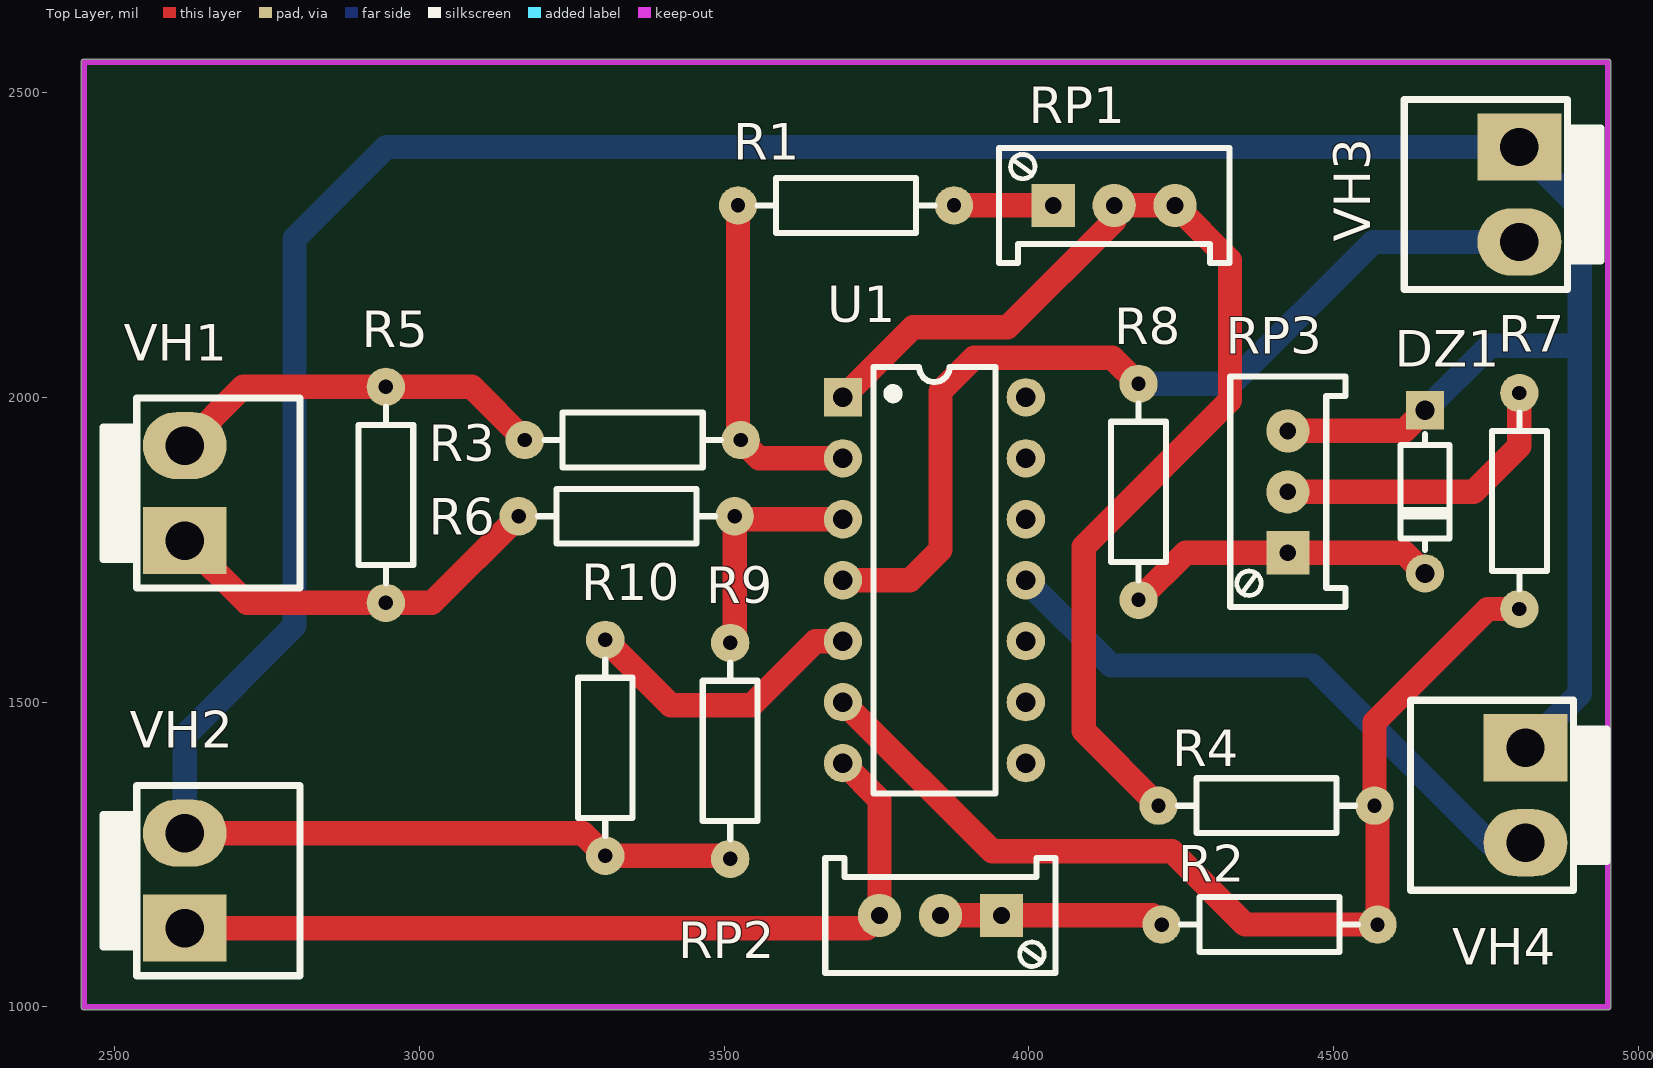
[diagram p0: Top Layer view]
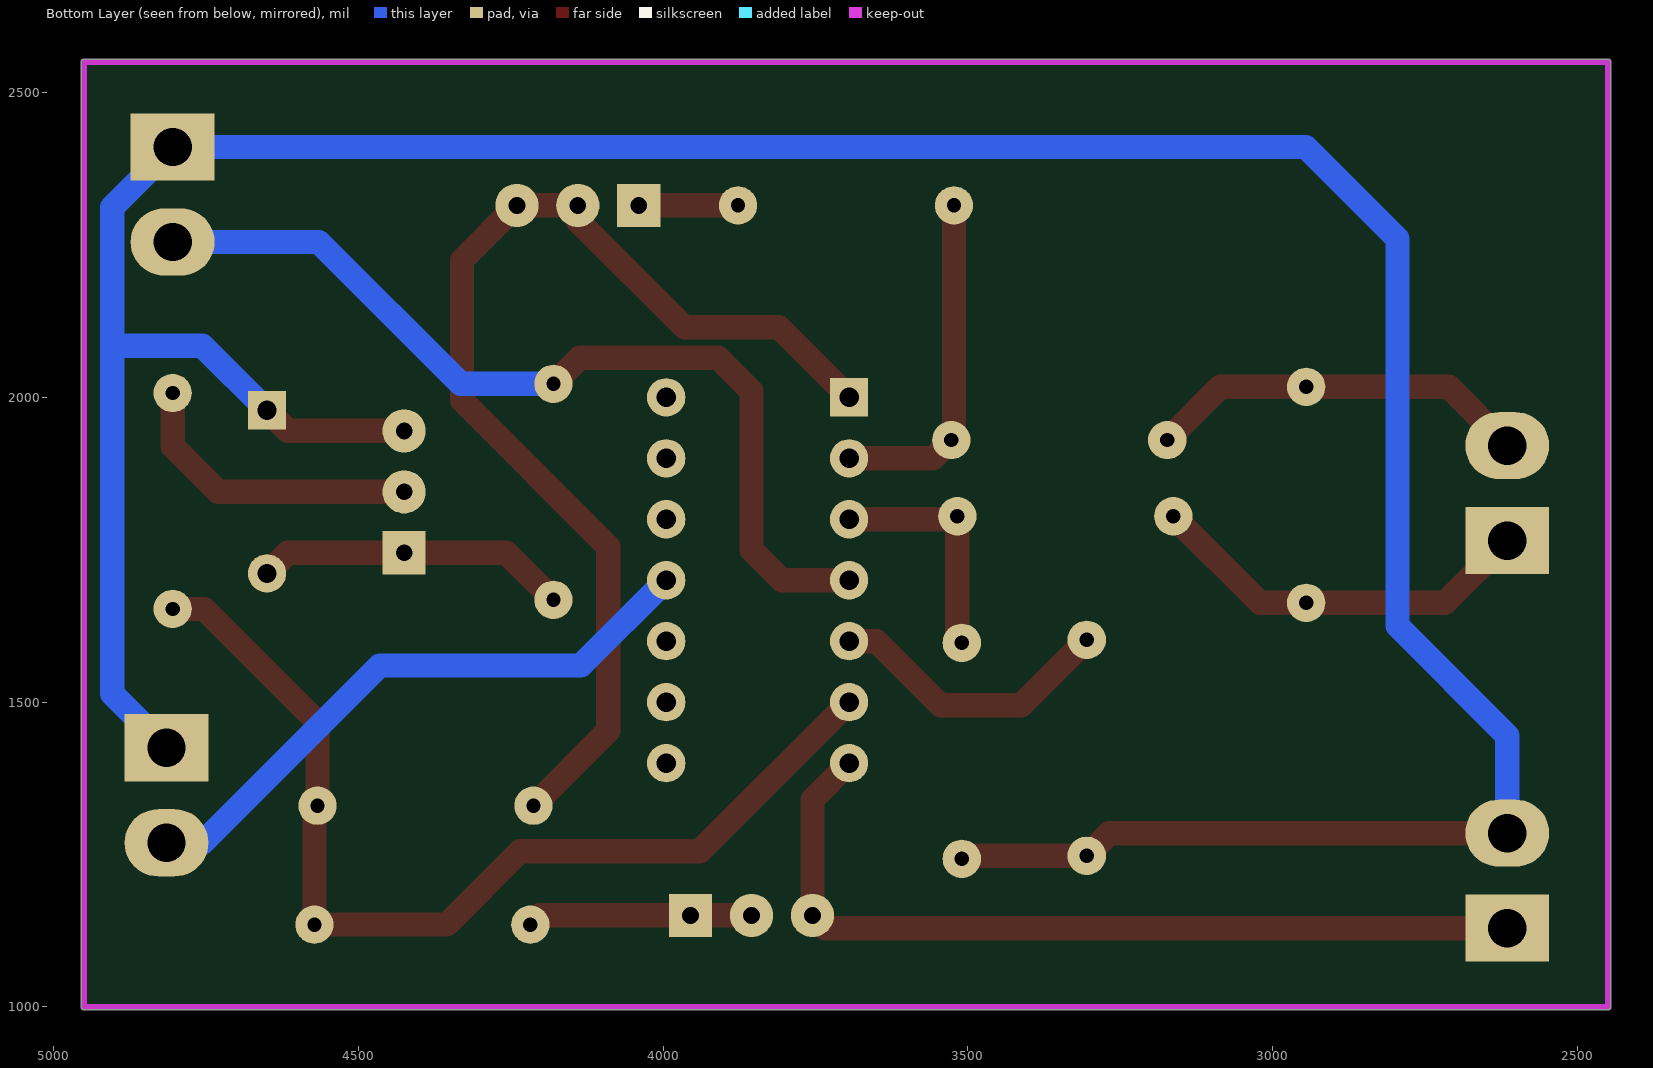
[diagram p1: Bottom Layer view, seen from below]
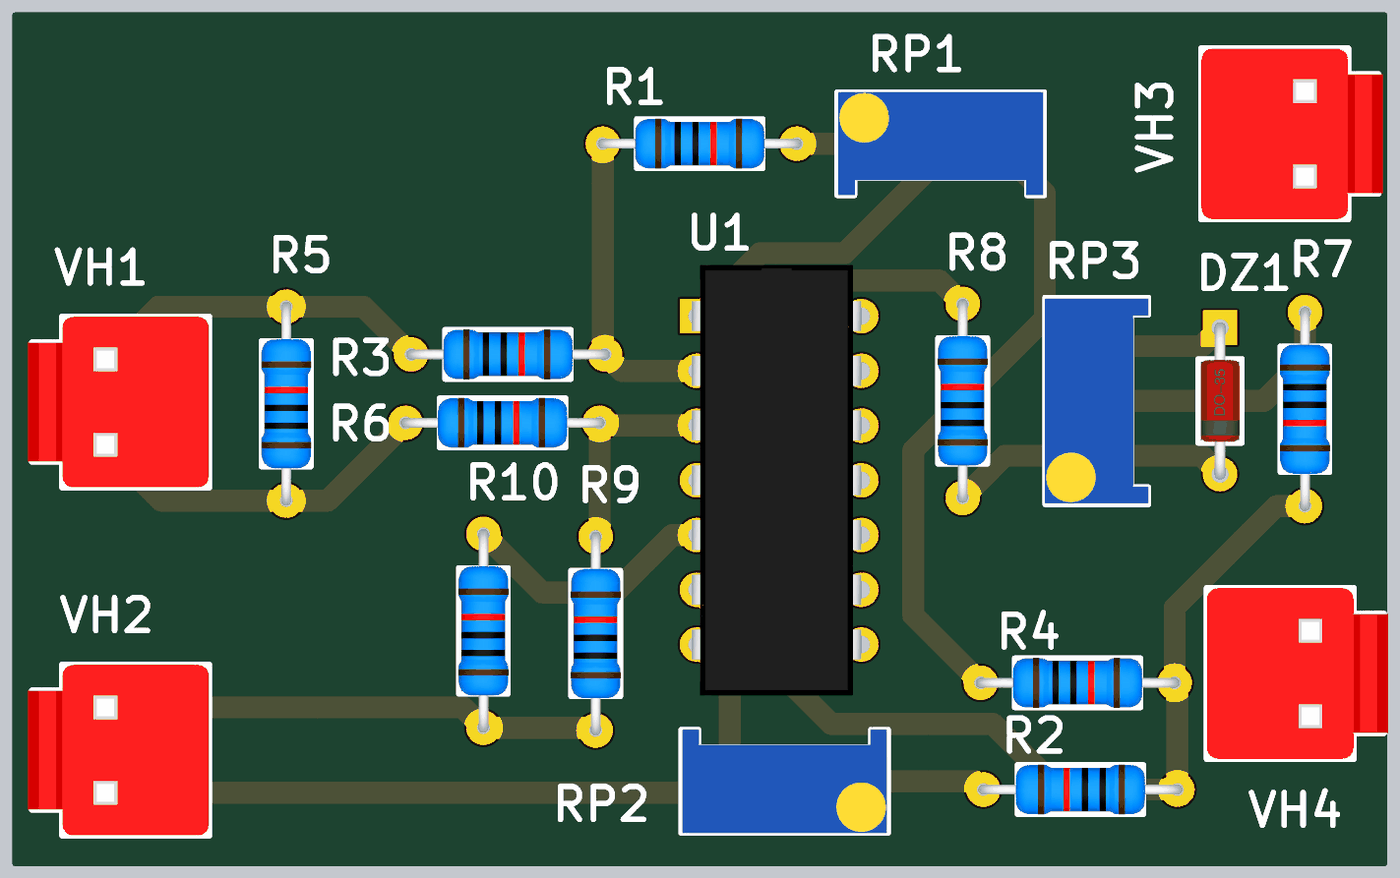
[diagram p2: 3D render of the assembled board from above, using the file's embedded part models]
# Altium PCB MISC80720.PcbDoc
Units mil, origin at the board's own origin, x right, y up, seen from the top; angles counter-clockwise.
Board outline 2510.03 x 1560.03 mil, 2 copper layers (Top Layer, Bottom Layer); 19 components, 15 nets, 53 pads, 0 vias.

## Layer stack, top to bottom (the 12.6 mil dielectric is the usual default, probably not edited)
Top Solder: solder mask 0.4, Solder Resist, Dk 3.5
Top Layer: signal copper 1.4
Dielectric 1: dielectric 12.6, FR-4, Dk 4.8
Bottom Layer: signal copper 1.4
Bottom Solder: solder mask 0.4, Solder Resist, Dk 3.5

## Board outline
2444.99,1000 ccw(c2450,1000) 2450,994.99 4950,994.99 ccw(c4950,1000) 4955.02,1000 4955.02,2550 ccw(c4950,2550) 4950,2555.01 2450,2555.01 ccw(c2450,2550) 2444.99,2550

## Design rules (kind name [scope] priority, off if disabled: settings)
Clearance [All] p1: gap=10
MinimumSolderMaskSliver [All] p1: minsoldermaskwidth=0
PolygonConnect [All] p1: connectstyle=Relief reliefconductorwidth=10 reliefentries=4 polygonreliefangle="90 Angle" airgapwidth=10
RoutingVias [All] p1: holewidth=28 width=50 viastyle="Through Hole" minholewidth=28 minwidth=50 maxholewidth=28 maxwidth=50
SilkToSilkClearance [All] p1: silktosilkclearance=0
SilkToSolderMaskClearance [IsPad] p1: minsilkscreentomaskgap=0 clearancetoexposedcopper=TRUE
SolderMaskExpansion [All] p1: expansion=4
Width [All] p1: maxlimit=40 minlimit=40 preferedwidth=40
27 further rules are at their usual default settings.

## Components (designator, comment, footprint, x,y, rotation, side; value= is the part's Value field where it differs from the comment)
DZ1 "6V2" DO-35 4650,1845 r270 top
R1 "9.1K" "RS 1/4W" 3700,2315 r0 top
R2 "22K" "RS 1/4W" 4395,1135 r180 top
R3 "10K" "RS 1/4W" 3350,1930 r0 top
R4 "10K" "RS 1/4W" 4390,1330 r0 top
R5 "500" "RS 1/4W" 2945,1840 r90 top
R6 "10K" "RS 1/4W" 3340,1805 r0 top
R7 "10K" "RS 1/4W" 4805,1830 r270 top
R8 "750" "RS 1/4W" 4180,1845 r90 top
R9 "10K" "RS 1/4W" 3510,1420 r90 top
R10 "3.9K" "RS 1/4W" 3305,1425 r90 top
RP1 "2K" 3296W 4140,2315 r0 top
RP2 "5K" 3296W 3855,1150 r180 top
RP3 "2K" 3296W 4425,1845 r90 top
U1 "LM124AD" DIP14 3695,2000 r0 top
VH1 "VH2" VH3.96-2A 2615,1765 r90 top
VH2 "VH2" VH3.96-2A 2615,1129.09 r90 top
VH3 "VH2" VH3.96-2A 4805,2410.91 r270 top
VH4 "VH2" VH3.96-2A 4815,1425 r270 top

## Footprints (in the part's own frame and the unit in brackets; to place one, negate y for a bottom-side part, rotate by r counter-clockwise, add the part's x,y. Pads: shape width x height; smd on the part's side, far side on the other; paste and mask are expansions set on the pad)
3296W [mm] "Precise Multi-Winding Adjustable Resistor"
  rect 1.8x1.8 hole 0.7: 1(-2.54,0)
  round 1.8 hole 0.7: 2(0,0) 3(2.54,0)
  silkscreen extent -4.8,-2.4 4.8,2.4, body extent -4.75,-2.4 4.75,2.4, height 11.52
DIP14 [mm]
  rect 1.6x1.6 hole 0.813: 1(0,0)
  round 1.6 hole 0.813: 2(0,-2.54) 3(0,-5.08) 4(0,-7.62) 5(0,-10.16) 6(0,-12.7) 7(0,-15.24) 8(7.62,-15.24) 9(7.62,-12.7) 10(7.62,-10.16) 11(7.62,-7.62) 12(7.62,-5.08) 13(7.62,-2.54) 14(7.62,0)
  silkscreen extent 1.27,-16.51 6.35,1.27, body extent -0.25,-17.62 7.62,2.38, height 5.1
DO-35 [mm] "1.8*6.8mm(直径，脚距）"
  rect 1.6x1.6 hole 0.8: 1(-3.4,0)
  round 1.6 hole 0.8: 2(3.4,0)
  silkscreen extent -2.41,-1.02 2.41,1.02, body extent -3.65,-0.9 3.65,0.9, height 1.85
"RS 1/4W" [mm] "直插色环电阻，脚距9mm，直径2.3mm"
  round 1.6 hole 0.6: 1(-4.5,0) 2(4.5,0)
  silkscreen extent -3.68,-1.14 3.68,1.14, body extent -4.72,-1.16 4.73,1.16, height 2.32
VH3.96-2A [mm]
  rect 2.8x3.5 hole 1.6: 1(0,0)
  oval 2.8x3.5 hole 1.6: 2(3.96,0)
  silkscreen extent -1.98,-4.8 5.94,3.4, body extent -1.98,-4.8 5.94,3.6, height 14.6

## Part data
DZ1: library part 1N4106, "12V/0.5W Zener diode"
R1 R2 R3 R4 R5 R6 R7 R8 R9 R10: library part R-S, "Color-band resistor"
RP1 RP2 RP3: library part RP, "Single-gang potentiometer"
U1: "Low-Power Quad Operational Amplifier"

## Nets (pads, with @x,y where several pads share a name; then routed paths per layer and width w, separated by ;. In a path a pad name is that pad's centre, name@x,y a point inside that pad or via, vN(x,y) a via of type N, cw(c..) or ccw(c..) an arc to the next point about the centre after c; other vN are vias at no path point)
+12V: R8.2 U1.4 VH3.2 | length 1527.7
  Top Layer w40: U1.4 3805,1700 3855,1750 3855,2010 3910,2065 4137.17,2065 R8.2
  Bottom Layer w40: R8.2 4332.17,2022.17 4565,2255 VH3.2
-12V: U1.11 VH4.2 | length 998.5
  Bottom Layer w40: U1.11 4135,1560 4465,1560 4755.91,1269.09 VH4.2
GND: DZ1.1 R9.1 R10.1 RP3.3 VH2.2 VH3.1 VH4.1 | length 5635.1
  Top Layer w40: VH2.2 3267.83,1285 R10.1 3505,1247.83 R9.1 ; RP3.3 4616.14,1945 DZ1.1
  Bottom Layer w40: VH2.2 2615,1445 2795,1625 2795,2260 2945.91,2410.91 VH3.1 4903.9,2312.01 4903.9,2085 ; DZ1.1 4756.14,2085 4903.9,2085 ; VH4.1 4903.9,1513.9 4903.9,2085
NetDZ1_2: DZ1.2 R8.1 RP3.1 | length 516
  Top Layer w40: R8.1 4257.17,1745 RP3.1 4616.14,1745 DZ1.2
NetR1_1: R1.1 R3.2 U1.2 | length 567.1
  Top Layer w40: R1.1 3522.83,1934.33 R3.2 3557.17,1900 U1.2
NetR1_2: R1.2 RP1.1 | length 162.8
  Top Layer w40: R1.2 RP1.1
NetR2_1: R2.1 R4.2 R7.2 U1.6 | length 1677.3
  Top Layer w40: U1.6 3940,1255 4235,1255 4355,1135 R2.1 4572.17,1325 R4.2 4567.17,1467.17 4752.83,1652.83 R7.2
NetR2_2: R2.2 RP2.1 RP2.2 | length 369
  Top Layer w40: RP2.2 RP2.1 4202.83,1150 R2.2
NetR3_1: R3.1 R5.2 VH1.2 | length 633.8
  Top Layer w40: VH1.2 2711.26,2017.17 R5.2 3085.67,2017.17 R3.1
NetR4_1: R4.1 RP1.2 RP1.3 U1.1 | length 1862.7
  Top Layer w40: U1.1 3810,2115 3965,2115 4140,2290 RP1.2 RP1.3 4330,2225 4330,1995 4090,1755 4090,1452.83 R4.1
NetR5_1: R5.1 R6.1 VH1.1 | length 649
  Top Layer w40: VH1.1 2717.17,1662.83 R5.1 3020.67,1662.83 R6.1
NetR6_2: R6.2 R9.2 U1.3 | length 390.7
  Top Layer w40: R9.2 3517.17,1604.33 R6.2 3522.17,1800 U1.3
NetR7_1: R7.1 RP3.2 | length 498.2
  Top Layer w40: RP3.2 4730,1845 4805,1920 R7.1
NetR10_2: R10.2 U1.5 | length 477.9
  Top Layer w40: R10.2 3412.17,1495 3545,1495 3650,1600 U1.5
NetRP2_3: RP2.3 U1.7 VH2.1 | length 1423.5
  Top Layer w40: VH2.1 3734.09,1129.09 RP2.3 3755,1340 U1.7
pads on no net: U1.8 U1.9 U1.10 U1.12 U1.13 U1.14

## Keep-outs
Keep-Out Layer:
  lines w10: 2450,2135 2450,2550 4950,2550 4950,1000 2450,1000 2450,2215